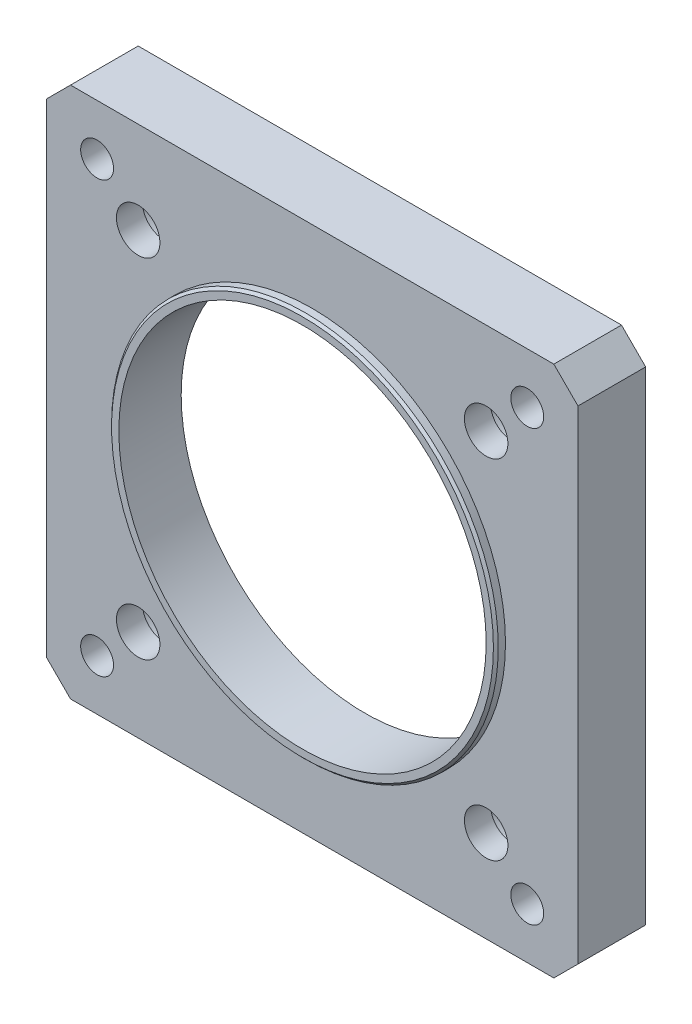
from build123d import *

# Parameters (mm, degrees)
SKETCH_1_W                     = 110
SKETCH_1_H                     = 110
EXTRUDE_1_DEPTH                = 14
SKETCH_2_R                     = 40
SKETCH_2_R_2                   = 38
EXTRUDE_2_DEPTH                = 2
SKETCH_3_R                     = 38
CUT_EXTRUDE_1_DEPTH            = 80.031639234
SKETCH_4_R                     = 42.5
CUT_EXTRUDE_2_DEPTH            = 3.1
HOLE_WIZARD_M8_1_D             = 6.8
HOLE_WIZARD_M8_1_2_D           = 9
HOLE_WIZARD_M8_1_2_CBORE_D     = 15
HOLE_WIZARD_M8_1_2_CBORE_DEPTH = 8.6
CHAMFER_1_SIZE                 = 5
CHAMFER_2_SIZE                 = 0.5


with BuildPart() as part:
    # 草图1 → 凸台-拉伸1 (new body)
    with BuildSketch(Plane.XY):
        Rectangle(SKETCH_1_W, SKETCH_1_H)
    extrude(amount=EXTRUDE_1_DEPTH)

    # 草图2 → 凸台-拉伸2 (add)
    with BuildSketch(Plane.XY.offset(14)):
        with Locations(Location((0, 0, 0), (0, 0, 180))):
            Circle(SKETCH_2_R)
        Circle(SKETCH_2_R_2, mode=Mode.SUBTRACT)
    extrude(amount=EXTRUDE_2_DEPTH)

    # 草图3 → 切除-拉伸1 (cut, through all)
    with BuildSketch(Plane.XY.offset(14)):
        Circle(SKETCH_3_R)
    extrude(amount=-CUT_EXTRUDE_1_DEPTH, mode=Mode.SUBTRACT)

    # 草图4 → 切除-拉伸2 (cut)
    with BuildSketch(Plane(origin=(0, 0, 0), x_dir=(-1, 0, 0), z_dir=(0, 0, -1))):
        Circle(SKETCH_4_R)
    extrude(amount=-CUT_EXTRUDE_2_DEPTH, mode=Mode.SUBTRACT)

    # Hole Wizard M8 _1 (through all)
    with Locations(Plane(origin=(0, 0, 0), x_dir=(-1, 0, 0), z_dir=(0, 0, -1))):
        with Locations((-44.5, 44.5), (0, 0), (44.5, 44.5), (-44.5, -44.5), (44.5, -44.5)):
            Hole(HOLE_WIZARD_M8_1_D / 2)

    # Hole Wizard M8 _1 2 (through all)
    with Locations(Plane(origin=(0, 0, 0), x_dir=(-1, 0, 0), z_dir=(0, 0, -1))):
        with Locations((36, -36), (36, 36), (-36, -36), (-36, 36)):
            CounterBoreHole(HOLE_WIZARD_M8_1_2_D / 2, HOLE_WIZARD_M8_1_2_CBORE_D / 2, HOLE_WIZARD_M8_1_2_CBORE_DEPTH)

    # 倒角1
    chamfer_1_edges = [part.edges().sort_by_distance(p)[0] for p in [
        (55, -55, 7),
        (-55, -55, 7),
        (-55, 55, 7),
        (55, 55, 7),
    ]]
    chamfer(chamfer_1_edges, length=CHAMFER_1_SIZE)

    # 倒角2
    chamfer_2_edges = [part.edges().sort_by_distance(p)[0] for p in [
        (40, 0, 16),
        (42.5, 0, 0),
    ]]
    chamfer(chamfer_2_edges, length=CHAMFER_2_SIZE)


solid = part.part
